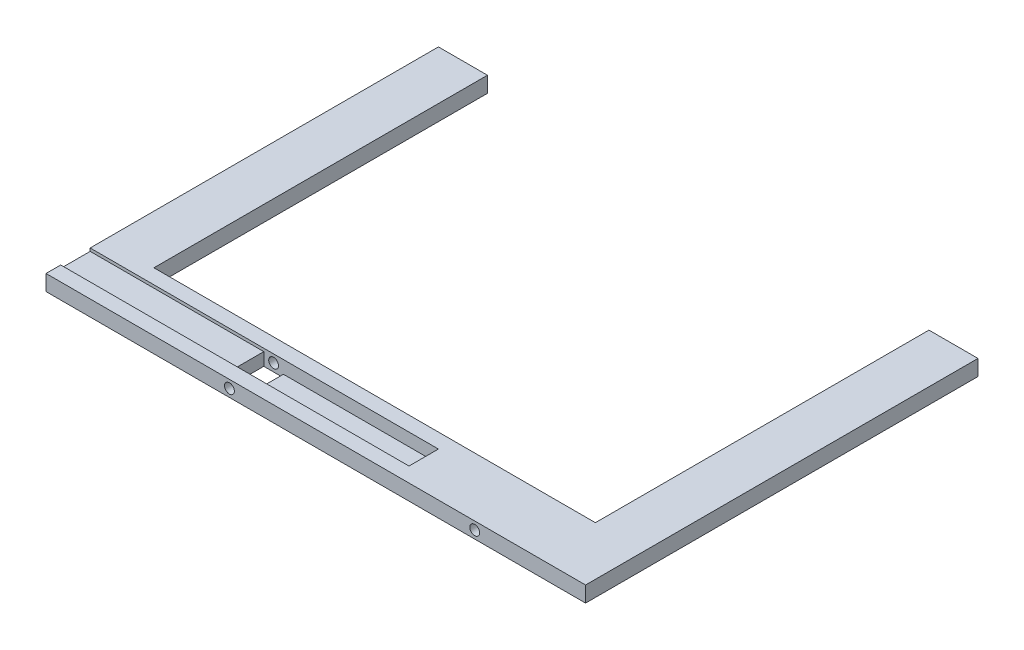
from build123d import *

# Parameters (mm, degrees)
BOSS_EXTRUDE1_DEPTH            = 30
SKETCH2_W                      = 8
SKETCH2_H                      = 30
BOSS_EXTRUDE2_DEPTH            = 8
SKETCH3_W                      = 8
SKETCH3_H                      = 16
BOSS_EXTRUDE3_DEPTH            = 15
SKETCH4_W                      = 45
SKETCH4_H                      = 16
BOSS_EXTRUDE4_DEPTH            = 195
SKETCH5_W                      = 45
SKETCH5_H                      = 16
BOSS_EXTRUDE5_DEPTH            = 347
SKETCH6_W                      = 347
SKETCH6_H                      = 30
CUT_EXTRUDE1_DEPTH             = 3
SKETCH7_W                      = 30
SKETCH7_H                      = 5
CUT_EXTRUDE2_DEPTH             = 150
SKETCH8_W                      = 30
SKETCH8_H                      = 13
CUT_EXTRUDE3_DEPTH             = 20
SKETCH9_W                      = 150
SKETCH9_H                      = 30
CUT_EXTRUDE4_DEPTH             = 5
SKETCH10_W                     = 550
SKETCH10_H                     = 16
BOSS_EXTRUDE6_DEPTH            = 355
SKETCH11_W                     = 450
SKETCH11_H                     = 340
CUT_EXTRUDE5_DEPTH             = 681.261714342
F_10_0_10_DIAMETER_HOLE1_D     = 10
F_10_0_10_DIAMETER_HOLE1_DEPTH = 20
F_10_0_10_DIAMETER_HOLE2_D     = 10
F_10_0_10_DIAMETER_HOLE2_DEPTH = 15
F_10_0_10_DIAMETER_HOLE3_D     = 10
F_10_0_10_DIAMETER_HOLE3_DEPTH = 355


with BuildPart() as part:
    # Sketch1 → Boss-Extrude1 (new body)
    with BuildSketch(Plane(origin=(0, 0, -45), x_dir=(-1, 0, 0), z_dir=(0, 0, -1))):
        Polygon((-355, -8), (-347, -8), (-355, 0), align=None)
    extrude(amount=-BOSS_EXTRUDE1_DEPTH)

    # Sketch2 → Boss-Extrude2 (add)
    with BuildSketch(Plane.XZ.offset(8)):
        with Locations((351, -30)):
            Rectangle(SKETCH2_W, SKETCH2_H)
    extrude(amount=BOSS_EXTRUDE2_DEPTH)

    # Sketch3 → Boss-Extrude3 (add)
    with BuildSketch(Plane.XY.offset(-15)):
        with Locations((351, -8)):
            Rectangle(SKETCH3_W, SKETCH3_H)
    extrude(amount=BOSS_EXTRUDE3_DEPTH)

    # Sketch4 → Boss-Extrude4 (add)
    with BuildSketch(Plane(origin=(355, 0, 0), x_dir=(0, 0, -1), z_dir=(1, 0, 0))):
        with Locations((22.5, -8)):
            Rectangle(SKETCH4_W, SKETCH4_H)
    extrude(amount=BOSS_EXTRUDE4_DEPTH)

    # Sketch5 → Boss-Extrude5 (add)
    with BuildSketch(Plane.ZY.offset(-347)):
        with Locations((-22.5, -8)):
            Rectangle(SKETCH5_W, SKETCH5_H)
    extrude(amount=BOSS_EXTRUDE5_DEPTH)

    # Sketch6 → Cut-Extrude1 (cut)
    with BuildSketch(Plane(origin=(0, 0, 0), x_dir=(-1, 0, 0), z_dir=(0, 1, 0))):
        with Locations((-173.5, -30)):
            Rectangle(SKETCH6_W, SKETCH6_H)
    extrude(amount=-CUT_EXTRUDE1_DEPTH, mode=Mode.SUBTRACT)

    # Sketch7 → Cut-Extrude2 (cut)
    with BuildSketch(Plane(origin=(347, 0, 0), x_dir=(0, 0, -1), z_dir=(1, 0, 0))):
        with Locations((30, -5.5)):
            Rectangle(SKETCH7_W, SKETCH7_H)
    extrude(amount=-CUT_EXTRUDE2_DEPTH, mode=Mode.SUBTRACT)

    # Sketch8 → Cut-Extrude3 (cut)
    with BuildSketch(Plane(origin=(197, 0, 0), x_dir=(0, 0, -1), z_dir=(1, 0, 0))):
        with Locations((30, -9.5)):
            Rectangle(SKETCH8_W, SKETCH8_H)
    extrude(amount=-CUT_EXTRUDE3_DEPTH, mode=Mode.SUBTRACT)

    # Sketch9 → Cut-Extrude4 (cut)
    with BuildSketch(Plane(origin=(0, -8, 0), x_dir=(-1, 0, 0), z_dir=(0, 1, 0))):
        with Locations((-272, -30)):
            Rectangle(SKETCH9_W, SKETCH9_H)
    extrude(amount=-CUT_EXTRUDE4_DEPTH, mode=Mode.SUBTRACT)

    # Sketch10 → Boss-Extrude6 (add)
    with BuildSketch(Plane(origin=(0, 0, -45), x_dir=(-1, 0, 0), z_dir=(0, 0, -1))):
        with Locations((-275, -8)):
            Rectangle(SKETCH10_W, SKETCH10_H)
    extrude(amount=BOSS_EXTRUDE6_DEPTH)

    # Sketch11 → Cut-Extrude5 (cut, through all)
    with BuildSketch(Plane(origin=(0, 0, 0), x_dir=(-1, 0, 0), z_dir=(0, 1, 0))):
        with Locations((-275, -230)):
            Rectangle(SKETCH11_W, SKETCH11_H)
    extrude(amount=-CUT_EXTRUDE5_DEPTH, mode=Mode.SUBTRACT)

    # Ø10.0 (10) Diameter Hole1
    with Locations(Plane.XY):
        with Locations((437, -8)):
            Hole(F_10_0_10_DIAMETER_HOLE1_D / 2, depth=F_10_0_10_DIAMETER_HOLE1_DEPTH)

    # Ø10.0 (10) Diameter Hole2
    with Locations(Plane.XY):
        with Locations((187, -8)):
            Hole(F_10_0_10_DIAMETER_HOLE2_D / 2, depth=F_10_0_10_DIAMETER_HOLE2_DEPTH)

    # Ø10.0 (10) Diameter Hole3
    with Locations(Plane.XY.offset(-45)):
        with Locations((187, -8)):
            Hole(F_10_0_10_DIAMETER_HOLE3_D / 2, depth=F_10_0_10_DIAMETER_HOLE3_DEPTH)


solid = part.part
